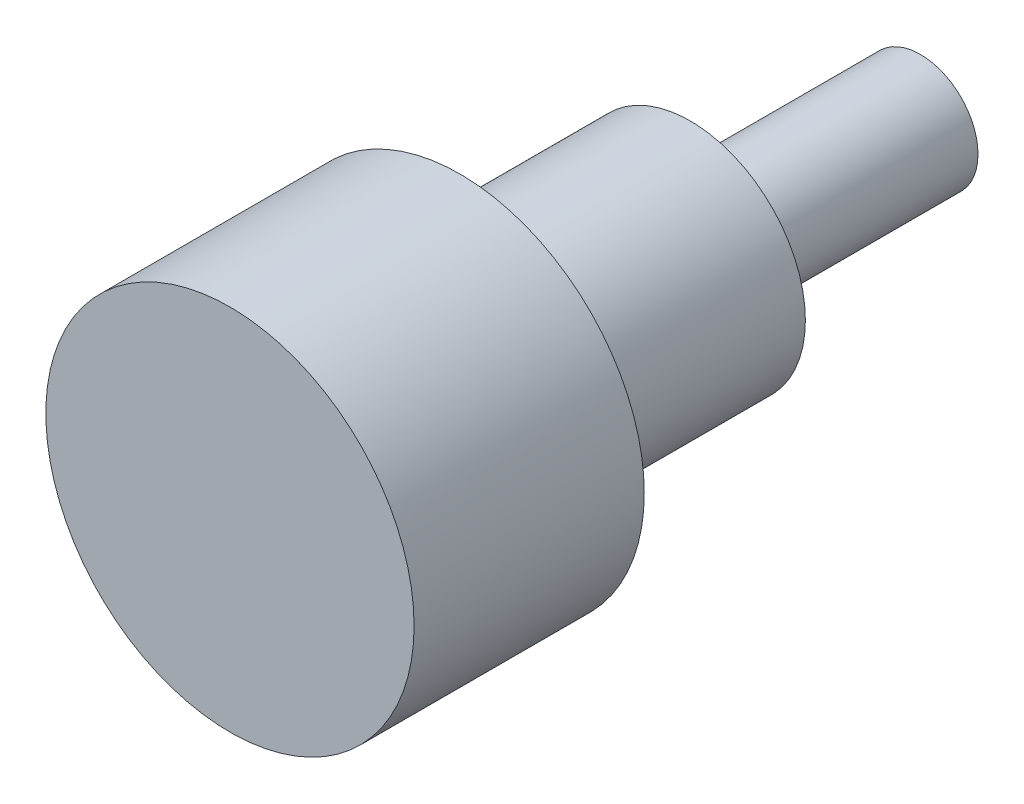
from build123d import *

# Parameters (mm, degrees)
SKETCH1_R           = 2.5
BOSS_EXTRUDE1_DEPTH = 10
SKETCH2_R           = 5
BOSS_EXTRUDE2_DEPTH = 10
SKETCH3_R           = 8
BOSS_EXTRUDE3_DEPTH = 10


with BuildPart() as part:
    # Sketch1 → Boss-Extrude1 (new body)
    with BuildSketch(Plane.XY):
        Circle(SKETCH1_R)
    extrude(amount=BOSS_EXTRUDE1_DEPTH)

    # Sketch2 → Boss-Extrude2 (add)
    with BuildSketch(Plane.XY.offset(10)):
        Circle(SKETCH2_R)
    extrude(amount=BOSS_EXTRUDE2_DEPTH)

    # Sketch3 → Boss-Extrude3 (add)
    with BuildSketch(Plane.XY.offset(20)):
        Circle(SKETCH3_R)
    extrude(amount=BOSS_EXTRUDE3_DEPTH)


solid = part.part
